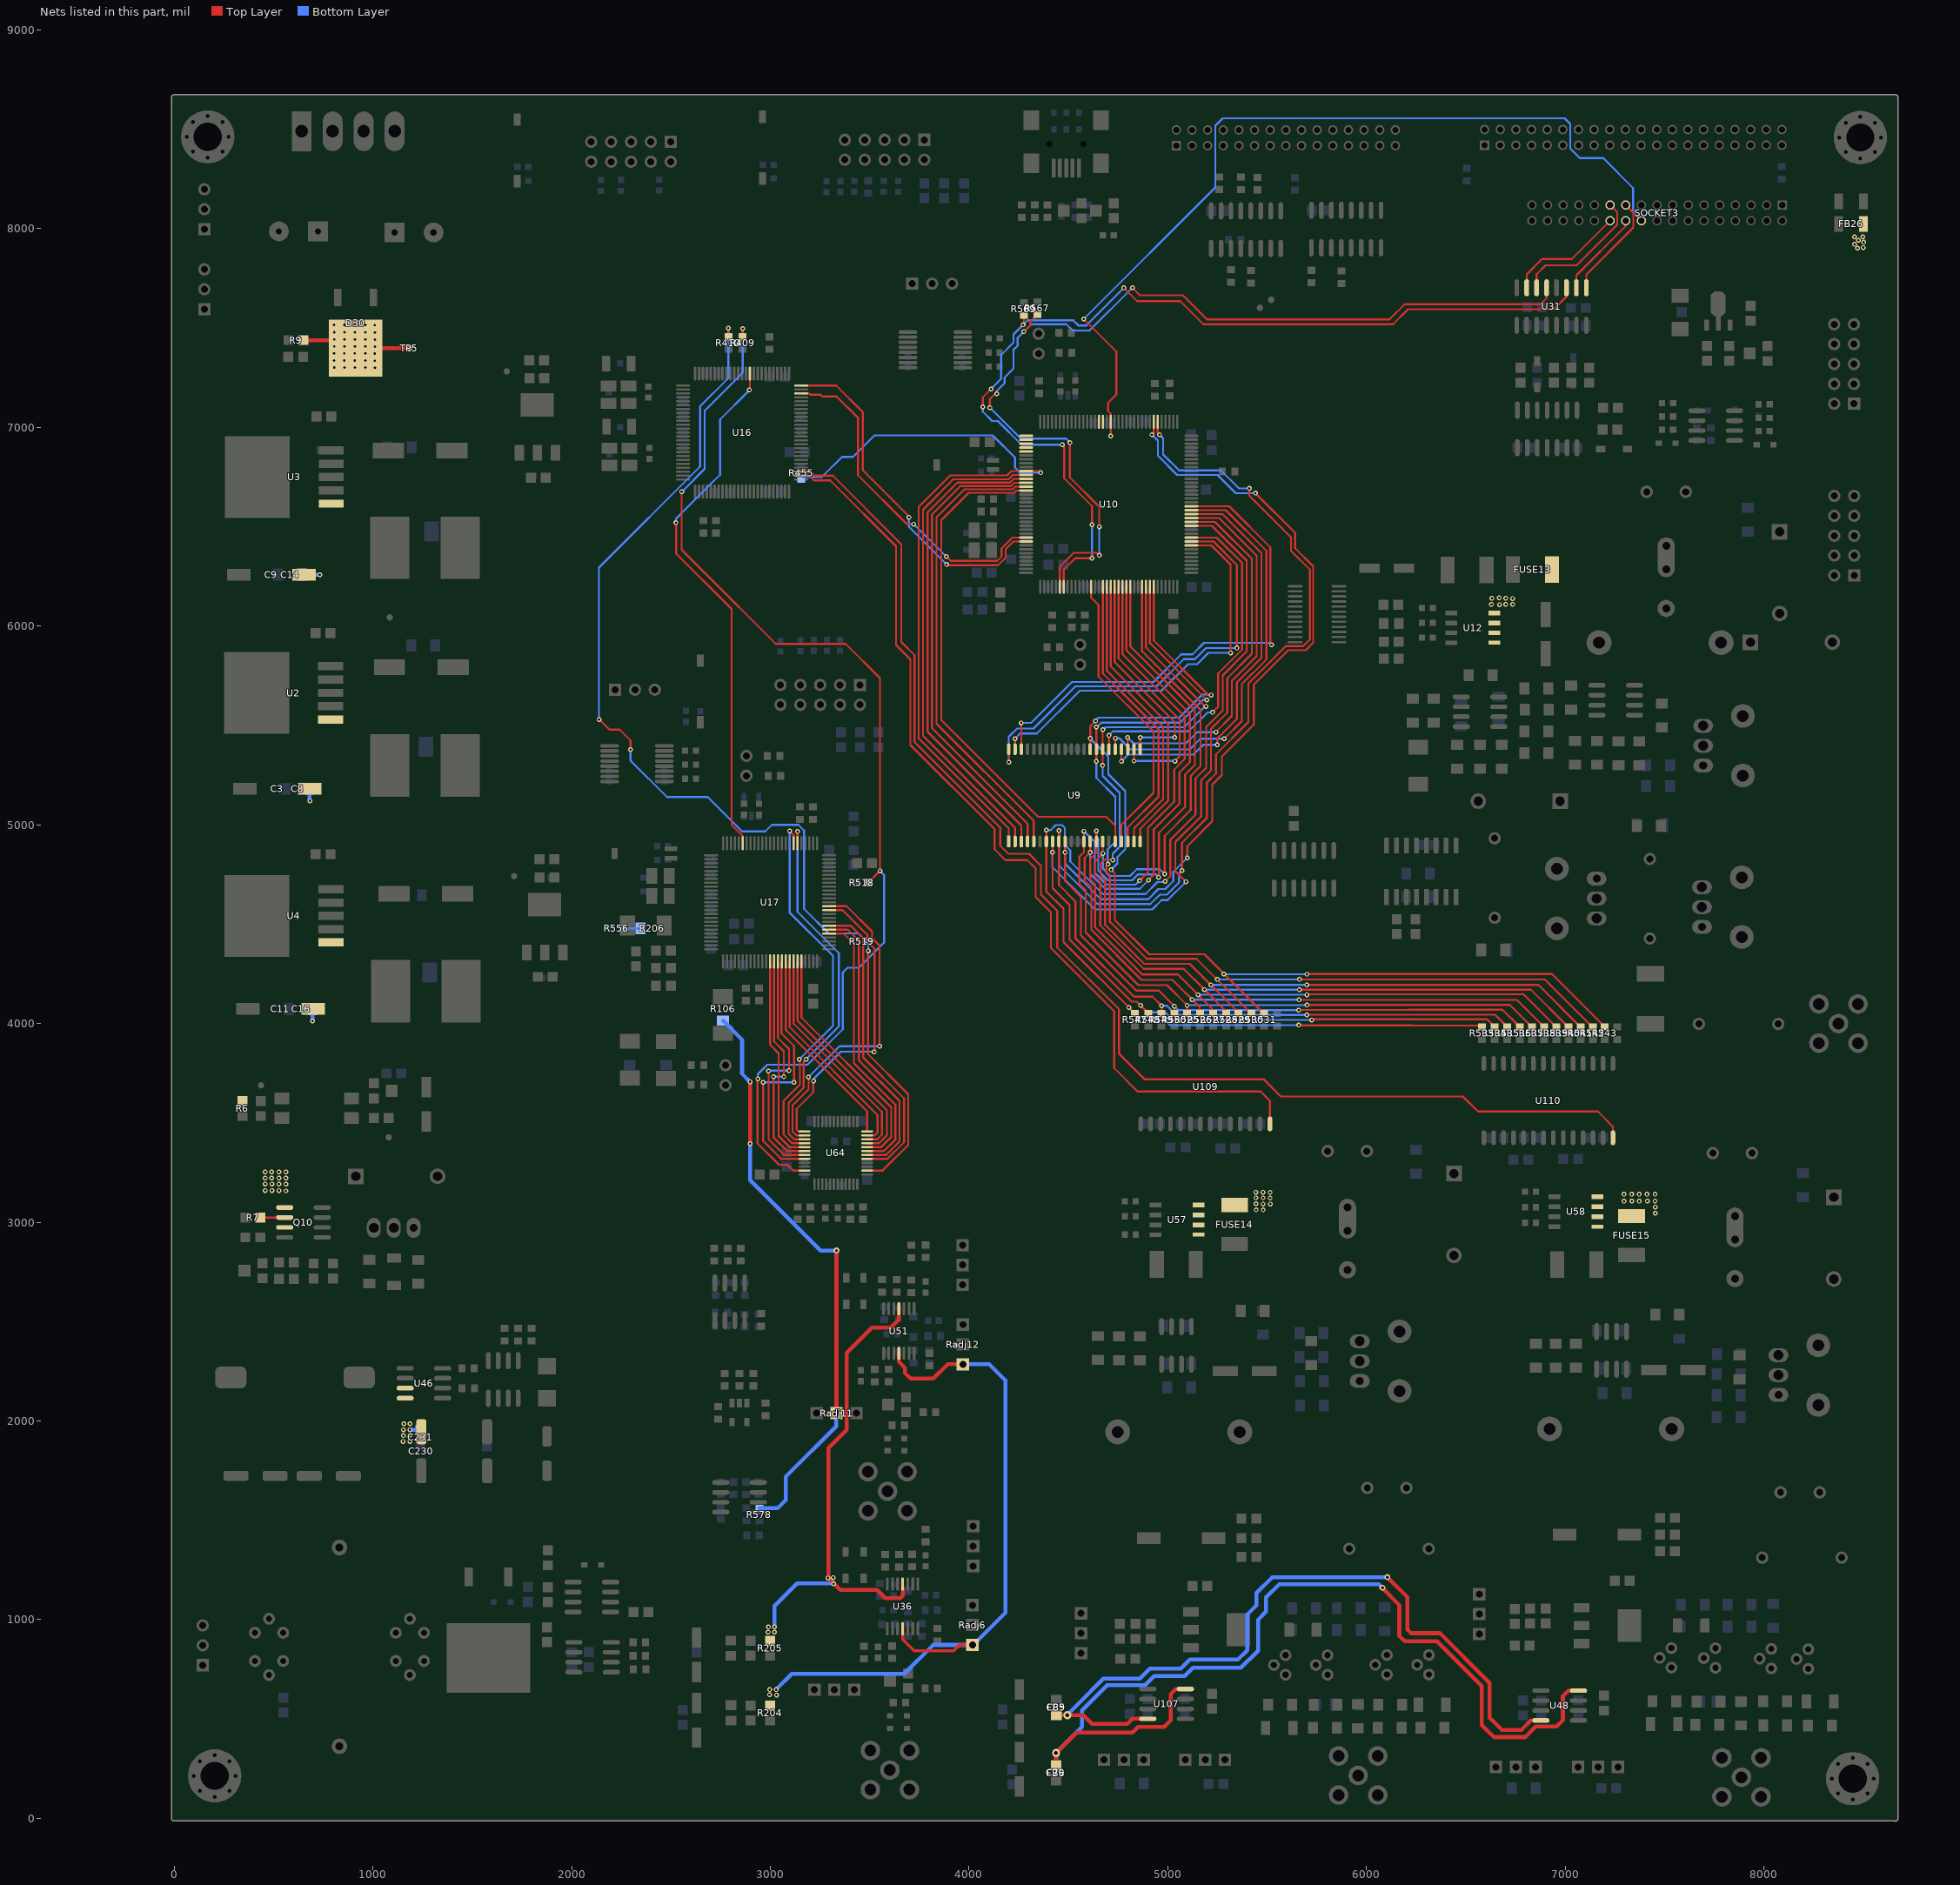
[diagram p0: the nets of this part, all layers, seen from the top]
# Altium PCB MISC82309.PcbDoc (part 6 of 14)
Units mil, origin at the board's own origin, x right, y up, seen from the top; angles counter-clockwise.
Board outline 8687.03 x 8687.86 mil, 4 copper layers (Top Layer, GND, POWER, Bottom Layer); 747 components, 583 nets, 2530 pads, 1834 vias.

## Via types
v1: diameter 24, hole 12, Top Layer to Bottom Layer, 1799 vias
v2: diameter 30, hole 15, Top Layer to Bottom Layer, 26 vias
v3: diameter 40, hole 20, Top Layer to Bottom Layer, 9 vias

## Nets (pads, with @x,y where several pads share a name; then routed paths per layer and width w, separated by ;. In a path a pad name is that pad's centre, name@x,y a point inside that pad or via, vN(x,y) a via of type N, cw(c..) or ccw(c..) an arc to the next point about the centre after c; other vN are vias at no path point) (continued)
DAC_+12V: C89.2 FB5.2 U48.8 U107.8 | length 3887.1
  Top Layer w20: FB5.2@4439,519.61 v3(4494.61,519.61) ; v3@4499,519.61 4575.39,519.61 4619,476 4797,476 4823,502 U107.8@4895,502 ; v2(6105,1214) 6205,1114 6205,951 6224,932 6370,932 6620,682 6620,507 6648,479 ; 6638,489 6648,479 ; U48.8@6877.51,493 6827,493 6780,446 6681,446 6648,479
  Bottom Layer w20: C89.2@4450,520 4450.39,519.61 C89.2@4456,519.61 ; C89.2@4456,520 4493,520 4523.5,550.5 4550.5,577.5 4676,703 4859,703 4910,754 5066,754 5111,799 5353,799 5400,846 5400,1026 5446,1072 5446,1134 5526,1214 v2(6105,1214)
DAC_-12V: C79.2 FB6.2 U48.4 U107.4 | length 4832.5
  Top Layer w20: FB6.2@4438,266.39 v3@4438,328 ; v3@4438.5,328.5 4542,432 4822,432 4851,461 4982,461 5014,493 5014,625 5039,650 U107.4@5085,650 ; v2(6080,1161) 6080,1159 6165,1074 6165,918 6192,891 6355,891 6580,666 6580,470 6641,409 6798,409 6852,463 6957,463 6988,494 6988,616 7015,643 U48.4@7066.49,643
  Bottom Layer w20: C79.2@4435,278 C79.2@4438,281 ; C79.2@4439,277 4439,331 4569,461 4569,544 4696,671 4885,671 4931,717 5085,717 5126,758 5368,758 5454,844 5454,1000 5494,1040 5494,1112 5561,1179 6062,1179 v2(6080,1161)
  other v3: 4438,329
DAC_CLK_A: U16.52 U109.28 | length 4718.4
  Top Layer w10: U16.52@3155.24,6757.46 3196,6757.46 3220.03,6733.44 3301,6733.44 3633,6401.44 3633,5905 3705,5833 3705,5402 4128,4979 4128,4877 4182,4823 4293,4823 4335,4781 4335,4637 4412,4560 4412,4380 4730,4062 4730,3776 4848,3658 5467,3658 5514,3611 U109.28@5514,3515
DAC_CLK_B: U16.53 U110.28 | length 6426.9
  Top Layer w10: U16.53@3155.24,6777.15 3200.85,6777.15 3221,6757 3314,6757 3659,6412 3659,5920 3726,5853 3726,5417 4157,4986 4157,4895 4198,4854 4302,4854 4362,4794 4362,4650 4444,4568 4444,4383 4755,4072 4755,3848 4883,3720 5482,3720 5569,3633 6485,3633 6561,3557 7164,3557 7240,3481 U110.28@7240,3424.99
DC-IN: C3.1 C8.2 C9.1 C11.1 C14.2 C16.2 C230.2 C231.2 D30.4 FB26.1 FUSE13.1 FUSE14.1 FUSE15.1 Q10.1 Q10.2 Q10.3 R6.2 R7.2 R9.2 TP5.1 U2.1 U3.1 U4.1 U12.5 U12.6 U12.7 U12.8 U46.7 U46.8 U57.5 U57.6 U57.7 U57.8 U58.5 U58.6 U58.7 U58.8 | length 778.8
  Top Layer w10: R7.2@433.5,3024 Q10.2@556.51,3024
  Top Layer w20: R9.2@650.5,7439 D30.4@887,7439 ; D30.4@1012,7404 1017,7399 TP5.1@1183,7399
  Bottom Layer w20: C14.2@644,6259 v1@734,6259 ; v1@682,5126 C8.2@682,5181 ; v1@697,4018 C16.2@697,4068 ; v1@1188,1956 1238.5,1956 C231.2@1239,1956.5
  other v1: 1152,1897 1187,1897 1154,1926 1187,1929 1153,1956 1187,1956 1156,1986 1187,1986 7453,3045 5445,3062 5480,3062 7453,3077 5480,3092 5516,3092 5444,3094 7296,3106 7372,3106 7335,3107 7413,3107 7452,3107 5515,3122 5443,3123 5480,3123 7295,3141 7334,3141 7372,3141 7412,3141 7452,3141 5515,3150 5443,3151 5479,3151 562,3158 459,3160 492,3160 528,3160 527,3192 562,3192 459,3193 492,3193 459,3223 491,3223 527,3223 562,3223 459,3253 491,3253 527,3253 562,3253 697,4013 683,5121 6669,6108 6629,6109 6736,6109 6701,6110 6735,6139 6631,6140 6701,6140 6668,6142 733,6258 1011,7300 806,7301 857,7301 910,7301 963,7301 1010,7335 805,7336 856,7336 909,7336 962,7336 1010,7371 805,7372 856,7372 909,7372 962,7372 1011,7406 806,7407 857,7407 910,7407 963,7407 1011,7441 806,7442 857,7442 910,7442 963,7442 1011,7478 806,7479 857,7479 910,7479 963,7479 1010,7515 805,7516 856,7516 909,7516 962,7516 8471,7902 8499,7905 8456,7921 8501,7932 8475,7941 8456,7959 8497,7959
DET+12V: R204.2 Radj6.3 Radj12.3 U36.4 U51.4 | length 3610.8
  Top Layer w16: U36.4@3667,953.8 3667,900 3723,844 3923,844 3952,873 Radj6.3@4015,873
  Top Layer w20: U51.4@3647,2340.8 3647,2298 3678,2267 3678,2241 3706,2213 3820,2213 3892,2285 Radj12.3@3969,2285
  Bottom Layer w20: v1@3030.5,649.5 3108,727 3674,727 3820,873 Radj6.3@4017,873 4021,873 4183,1035 4183,2204 4102,2285 Radj12.3@3969,2285
  other v1: 3031,621 2996,622 2997,648 3030,648
DET-12V: R205.2 U36.11 U51.11 | length 2465.2
  Top Layer w20: v1@3320,1182 3352,1150 3538,1150 3579,1109 3654,1109 3666,1121 U36.11@3666,1161 ; v1@3320.5,1182.5 3292,1211 3292,1863 3385,1956 3385,2343 3511,2469 3606,2469 3647,2510 U51.11@3647,2565.2
  Bottom Layer w20: v1(3021,964) 3021,1069 3134,1182 v1@3316,1182
  other v1: 2989,938 3021,938 2991,963 3319,1181 3290,1210 3317,1212
DET_D0: U17.61 U64.37 | length 1548
  Top Layer w10: U64.37@3172.52,3457.27 3142.73,3457.27 3133,3467 3133,3571 3216,3654 3216,3712 v1(3217,3711) ; U17.61@3296.24,4570.63 3363.37,4570.63 3489,4445 3489,4412 3524,4377 v1@3524,3864 ; v1(3523,3857) 3524,3858 v1@3524,3864 ; v1@3523,3863 v1@3524,3864
  Bottom Layer w10: v1(3217,3711) 3217,3720 3355,3858 3524,3858 v1(3523,3857)
DET_D1: U17.62 U64.38 | length 1659.4
  Top Layer w10: U64.38@3172.52,3437.58 3131.42,3437.58 3112,3457 3112,3588 3193,3669 3193,3729 v1(3192,3730) ; U17.62@3296.24,4590.32 3384.68,4590.32 3512,4463 3512,4431 3550,4393 v1(3550,3886)
  Bottom Layer w10: v1(3192,3730) 3348,3886 v1(3550,3886)
DET_D2: U17.81 U64.39 | length 1862
  Top Layer w10: U17.81@3136.8,4907.24 3136.8,4965.8 v1(3137,4966) ; U64.39@3172.52,3417.9 3120.1,3417.9 3092,3446 3092,3601 3168,3677 3168,3808 v1(3180,3820)
  Bottom Layer w10: v1(3137,4966) 3137,4562 3345,4354 3345,3985 v1(3180,3820)
DET_D3: U17.82 U64.40 | length 1916.8
  Top Layer w10: v1(3097,4969) 3117.11,4948.89 U17.82@3117.11,4907.24 ; v1(3146,3820) 3149,3817 3149,3693 3067,3611 3067,3441 3109.79,3398.21 U64.40@3172.52,3398.21
  Bottom Layer w10: v1(3097,4969) 3097,4559 3315,4341 3315,3989 v1(3146,3820)
DET_D4: U17.38 U64.41 | length 1050.3
  Top Layer w10: U17.38@2999,4312.76 2999,3893 3042,3850 3042,3630 3042,3433.53 3097,3378.53 U64.41@3172.52,3378.53
DET_D5: U17.39 U64.42 | length 1147
  Top Layer w10: v1@3016,3737 v1(3016,3733) 3016,3680 3016,3426.84 3084,3358.84 U64.42@3172.52,3358.84 ; U17.39@3018.68,4312.76 3018.68,3910.32 3068,3861 v1(3068,3733)
  Bottom Layer w10: v1(3016,3733) v1(3068,3733)
DET_D6: U17.40 U64.43 | length 1234.3
  Top Layer w10: v1(2991,3761) 2991,3717 2991,3417.16 3069,3339.16 U64.43@3172.52,3339.16 ; U17.40@3038.37,4312.76 3038.37,3927.63 3094,3872 v1(3094,3763)
  Bottom Layer w10: v1(2991,3761) 2993,3763 v1(3094,3763)
DET_D7: U17.41 U64.44 | length 1332.2
  Top Layer w10: v1(2964,3704) 2964,3684 2964,3409.47 3054,3319.47 U64.44@3172.52,3319.47 ; U17.41@3058.06,4312.76 3056.28,4310.98 3056.28,3950.72 3119,3888 3119,3705 v1(3120,3704)
  Bottom Layer w10: v1(2964,3704) v1(3120,3704)
DET_D8: U17.42 U64.24 | length 1028.8
  Top Layer w10: U17.42@3077.74,4312.76 3077.74,3968.26 3487.48,3558.52 U64.24@3487.48,3457.27 U64.24@3490,3459.79
DET_D9: U17.43 U64.23 | length 1104.8
  Top Layer w10: U17.43@3099,4311.18 U17.43@3097.43,4312.76 3097.43,3981.57 3540,3539 3540,3452 3525.58,3437.58 U64.23@3487.48,3437.58
DET_D10: U17.44 U64.22 | length 1140.1
  Top Layer w10: U17.44@3117.11,4312.76 3117.11,3999.89 3562,3555 3562,3441 3538.9,3417.9 U64.22@3487.48,3417.9
DET_D11: U17.45 U64.21 | length 1177.2
  Top Layer w10: U17.45@3136.8,4312.76 3136.8,4014.2 3587,3564 3587,3438 3547.21,3398.21 U64.21@3487.48,3398.21
DET_D12: U17.46 U64.20 | length 1216.1
  Top Layer w10: U17.46@3158.26,4310.98 U17.46@3156.48,4312.76 3156.48,4030.52 3609,3578 3609,3429 3558.53,3378.53 U64.20@3487.48,3378.53
DET_D13: U17.55 U64.19 | length 1383.9
  Top Layer w10: U17.55@3296.24,4452.52 3369.48,4452.52 3420,4402 3420,3800 3630,3590 3630,3416 3572.84,3358.84 U64.19@3487.48,3358.84
DET_D14: U17.56 U64.18 | length 1458.3
  Top Layer w10: U17.56@3296.24,4472.2 3390.8,4472.2 3445,4418 3445,3816 3650,3611 3650,3406 3583.16,3339.16 U64.18@3487.48,3339.16
DET_D15: U17.57 U64.17 | length 1529.4
  Top Layer w10: U17.57@3296.24,4491.89 3405.11,4491.89 3468,4429 3468,3828 3673,3623 3673,3402 3590.47,3319.47 U64.17@3487.48,3319.47
DETECT-RST: U16.86 U17.95 | length 2654
  Top Layer w10: v1@2526,6520 2526,6365 2805,6086 2805,5000 2861.2,4943.8 U17.95@2861.2,4907.24 ; v1@2897.37,7190.37 U16.86@2897.37,7271.24
  Bottom Layer w10: v1(2525,6520) 2525,6540 2568,6583 2568,6583.47 2690.53,6706 2691,6706 2747,6762 2747,7040 v1(2895,7188)
DROP-CH_A: R206.1 R556.1 | length 82.7
  Bottom Layer w10: R556.1@2258.5,4479 2337,4479 R206.1@2340,4476
DROP-CH_B: R106.1 R578.1 Radj11.2 | length 2948.4
  Top Layer w20: v1(2898,3396) v1(2898,3707) ; Radj11.2@3333,2039 v2(3333,2858)
  Bottom Layer w20: R106.1@2762,4015 2858,3919 2858,3747 v1(2898,3707) ; v1(2898,3396) 2898,3212 3253,2857 v2@3332,2857 ; R578.1@2945,1560.5 3036.5,1560.5 3077,1601 3077,1719 3331,1973 Radj11.2@3331,2036
DROP_A: U10.27 U16.73 | length 1721.6
  Top Layer w10: U16.73@3155.24,7170.85 3195.15,7170.85 3202,7164 3253,7164 3261,7156 3333,7156 3440,7049 ; 3441,7049 3441,6760 3688,6513 v1(3721,6513) ; v1(3885,6350) v1@3886.5,6348.5 ; v1@3887,6349 3908,6328 4141.51,6328 4164,6350.49 4164,6391.04 4218.64,6445.68 U10.27@4287.65,6445.68
  Bottom Layer w10: v1@3723,6514 3723,6512 v1(3885,6350)
DROP_B: U10.28 U16.75 | length 1803.5
  Top Layer w10: U16.75@3155.24,7210.22 3331.78,7210.22 3464,7078 ; 3465,7078 3465,6785 v1@3703,6547 ; v1(3887,6310) 3887,6308 3885,6306 4146,6306 4184,6344 4184,6387 4222.99,6425.99 U10.28@4287.65,6425.99
  Bottom Layer w10: v1@3705,6548 3697,6540 3697,6500 3885,6312 3885,6306 3887,6308 v1(3887,6310)
  other v1: 3698,6547
ENC_A: R409.2 R518.2 U64.47 | length 5687.8
  Top Layer w10: v1(2554,6676) 2554,6384 2663,6275 3028,5910 3380,5910 3552,5738 v1(3552,4768.5) R518.2@3492.5,4709 ; R409.2@2861,7455.5 v1(2861,7497) ; v1@2936,3716 2936,3397 3044,3289 3086,3289 3114.58,3260.42 U64.47@3172.52,3260.42
  Bottom Layer w10: v1@2554.5,6675.5 2670,6791 2670,7084 2861,7275 v1(2861,7497) ; v1@2937,3717 v1(2937,3722) 2937,3745 2985,3793 3186.94,3793 3365,3971.06 3365,4257 3389,4281 3446,4281 3572,4407 3572,4748.5 v1(3552,4768.5)
ENC_B: R410.2 R519.2 U64.14 | length 5783.3
  Top Layer w10: v1@2140,5529 2190,5479 2242,5479 2297,5424 v1(2297,5379) ; v1(2789,7499) 2790,7498 R410.2@2790,7456.5 ; U64.14@3487.48,3260.42 3565.42,3260.42 3694,3389 3694,3644 3492,3846 3492,4365 v1(3493,4366)
  Bottom Layer w10: v1(2138,5529) 2138,6294 2647,6803 2647,7106 2789,7248 v1(2789,7499) ; v1(2297,5379) 2297,5323 2480,5140 2685,5140 2858,4967 2975,4967 3008,5000 3141,5000 3170,4971 3170,4577 3293,4454 3443.88,4454 3483.88,4414 R519.2@3492.5,4414 3493,4413.5 v1(3493,4366)
ENCODE_PA: R567.2 U10.42 U31.5 | length 4915
  Top Layer w10: v1(4105,7099) 4105,7143 4131,7169 v1(4139,7169) ; v1@4274,7480 v1(4276,7482) 4308,7514 4308,7533 R567.2@4332,7557 ; U10.42@4456.94,6197.65 4456.94,6298.94 4527,6369 4642,6369 v1(4655,6356) ; v1@4507,6918 4507,6749 4655,6601 v1(4655,6500) ; v1(4822,7703) 4860,7665 5076,7665 5198,7543 6115,7543 6192,7620 6876,7620 6906,7650 U31.5@6906,7702.49
  Bottom Layer w10: v1(4105,7099) 4261,6943 4488,6943 v1(4508,6923) ; v1(4139,7169) 4139,7183 4178.5,7222.5 4178.5,7250.5 4224,7296 4224,7391 4245,7412 4245,7451 v1(4276,7482) 4313,7519 4490,7519 4522,7487 4606,7487 v1(4822,7703) ; v1@4659,6352 v1(4655,6356) v1(4655,6500) v1@4659,6496
ENCODE_PB: R569.2 U10.43 U31.3 | length 4953.8
  Top Layer w10: v1(4069,7103) 4069,7151 v1(4111,7193) ; v1@4272,7509 v1(4272,7516) ; v1@4274,7516 4276,7518 R569.2@4276,7564.5 ; v1(4469,6913) 4479,6903 4479,6744 4619,6604 v1(4619,6510) ; U10.43@4476.62,6197.65 4476.62,6284.62 4534,6342 v1(4619,6342) ; v1(4779,7702) 4846,7635 5063,7635 5179,7519 6133,7519 6209,7595 6943,7595 7006,7658 U31.3@7006,7702.49
  Bottom Layer w10: v1(4069,7103) 4069,7079 4116,7032 4145,7032 4264,6913 4321,6913 v1(4469,6913) ; v1@4111,7194 4161,7244 4161,7364 4224,7427 4224,7468 v1(4272,7516) ; v1@4275.5,7512.5 4272,7509 v1(4272,7516) ; v1(4619,6342) v1(4619,6510) ; v1(4779,7702) 4590,7513 4550,7513 4524,7539 4295,7539 v1(4272,7516)
ENCODER_TRACK_AN: SOCKET3.24 U31.7 | length 599.3
  Top Layer w10: U31.7@6806,7702.49 6806,7770 6883,7847 7032.6,7847 SOCKET3.24@7225.86,8040.26
ENCODER_TRACK_AP: SOCKET3.23 U31.6 | length 690.6
  Top Layer w10: U31.6@6856,7702.49 6856,7771 6901,7816 7057,7816 7261.48,8020.48 7261.48,8083.38 SOCKET3.23@7225.86,8119
ENCODER_TRACK_BN: SOCKET3.21 U31.1 | length 530.6
  Top Layer w10: U31.1@7106,7702.49 7106,7769 7343,8006 7343,8080.6 SOCKET3.21@7304.6,8119
ENCODER_TRACK_BP: SOCKET3.22 U31.2 | length 440.7
  Top Layer w10: U31.2@7056,7702.49 7056,7765 7304.6,8013.6 SOCKET3.22@7304.6,8040.26
EPRINT-RST: SOCKET3.20 U10.126 | length 4442.7
  Top Layer w10: v1(4577,7545) 4741,7381 4741,7165 4700,7124 4700,7081 4712.84,7068.16 U10.126@4712.84,7028.35 4712.84,6957.16 v1(4713,6957)
  Bottom Layer w10: v1(4577,7545) 5239,8207 5239,8518 5276,8555 6997,8555 7025,8527 7025,8403 7073,8355 7191,8355 7342,8204 7342,8081.6 SOCKET3.20@7383.34,8040.26
FSMC_A0: R455.2 U9.1 U10.10 | length 3953.5
  Top Layer w10: U9.1@4200,4916 4200,4982 3747,5435 3747,6600 3905,6758 4191,6758 4213.32,6780.32 U10.10@4287.65,6780.32 4351.68,6780.32 v1(4360,6772)
  Bottom Layer w10: R455.2@3163,6751 3260,6751 3361,6852 3416,6852 3524,6960 4119,6960 4231,6848 4231,6798 4257,6772 v1(4360,6772)
FSMC_A1: U9.2 U10.11 | length 2454
  Top Layer w10: U9.2@4231.5,4916 4231.5,4985.5 3768,5449 3768,6586 3921,6739 4198.83,6739 4220.47,6760.64 U10.11@4287.65,6760.64
FSMC_A2: U9.3 U10.12 | length 2417.3
  Top Layer w10: U9.3@4262.99,4916 4262.99,4996.01 3792,5467 3792,6573 3941,6722 4205.88,6722 4224.83,6740.95 U10.12@4287.65,6740.95
FSMC_A3: U9.4 U10.13 | length 2385.5
  Top Layer w10: U10.13@4287.65,6721.27 4229.18,6721.27 4212.92,6705 3957,6705 3813,6561 3813,5487 4294.49,5005.51 U9.4@4294.49,4916
FSMC_A4: U9.5 U10.14 | length 2349.6
  Top Layer w10: U10.14@4287.65,6701.58 4233.54,6701.58 4219.96,6688 3977,6688 3836,6547 3836,5509 4325.98,5019.02 U9.5@4325.98,4916
FSMC_A5: U9.18 U10.15 | length 2670.5
  Top Layer w10: U10.15@4287.65,6681.9 4287.54,6682 4238,6682 4227,6671 4181.94,6671 3998,6671 3860,6533 3860,5527 4347,5040 4691,5040 4735.43,4995.57 U9.18@4735.43,4916
FSMC_A6: U9.19 U10.50 | length 1478.3
  Top Layer w10: U10.50@4614.42,6197.65 4614.42,6143.58 4652,6106 4652,5746 4928,5470 4928,5161 4766.93,4999.93 U9.19@4766.93,4916
FSMC_A7: U9.20 U10.53 | length 1461.5
  Top Layer w10: U10.53@4673.47,6197.65 4673.47,5761.53 4775,5660 4953,5482 4953,5141 4798.43,4986.43 U9.20@4798.43,4916
FSMC_A8: U9.21 U10.54 | length 1460.1
  Top Layer w10: U10.54@4693.16,6197.65 4693.16,5775.84 4977,5492 4977,5129 4829.92,4981.92 U9.21@4829.92,4916
FSMC_A9: U9.22 U10.55 | length 1459.6
  Top Layer w10: U10.55@4712.84,6197.65 4712.84,5798.16 5002,5509 5002,5121 4861.42,4980.42 U9.22@4861.42,4916
FSMC_A10: U9.23 U10.56 | length 1113.4
  Top Layer w10: U10.56@4732.53,6197.65 4732.53,5819.47 5036,5516 v1@5036,5442 ; U9.23@4861.42,5380.57 v1(4861.42,5439.42)
  Bottom Layer w10: v1(4861.42,5439.42) 4896,5439.42 v1(5034.58,5439.42)
FSMC_A11: U9.24 U10.57 | length 1281.1
  Top Layer w10: U10.57@4752.21,6197.65 4752.21,5837.79 5060,5530 5060,5344 v1(5036,5320) ; v1(4829.92,5321.08) U9.24@4829.92,5380.57
  Bottom Layer w10: v1(4829.92,5321.08) 5034.92,5321.08 v1(5036,5320)
FSMC_A12: U9.25 U10.87 | length 1923.2
  Top Layer w10: U9.25@4798.43,5380.57 v1(4798.43,5439.57) ; U10.87@5118.35,6544.1 5257.9,6544.1 5447,6355 5447,5849 5322,5724 5322,5548 v1@5240,5466
  Bottom Layer w10: v1(4798.43,5439.57) 4828,5410 5092,5410 5148,5466 5244,5466 v1(5243,5467)
FSMC_A13: U9.26 U10.88 | length 2076.6
  Top Layer w10: v1(4766.93,5319.07) U9.26@4766.93,5380.57 ; U10.88@5118.35,6563.79 5275.21,6563.79 5471,6368 5471,5840 5347,5716 5347,5532 5249,5434 v1(5249,5402)
  Bottom Layer w10: v1(4766.93,5319.07) 4800.86,5353 5129,5353 5178,5402 v1(5249,5402) v1@5256,5402
FSMC_A14: U9.27 U10.89 | length 2143.7
  Top Layer w10: U9.27@4735.43,5380.57 v1@4735.43,5436 ; U10.89@5118.35,6583.47 5291.53,6583.47 5496,6379 5496,5832 5373,5709 5373,5522 v1(5284,5433)
  Bottom Layer w10: v1(4737,5436) 4755,5436 4811,5380 5111,5380 5164,5433 v1(5284,5433)
FSMC_A15: U9.42 U10.90 | length 2538.4
  Top Layer w10: U9.42@4262.99,5380.57 v1(4262.99,5512.99) ; U10.90@5118.35,6603.16 5308.84,6603.16 5516,6396 5516,5912 v1(5522,5906)
  Bottom Layer w10: v1(4262.99,5512.99) 4311.99,5512.99 4518,5719 4928,5719 5067,5858 5124,5858 5182,5916 5512,5916 v1(5522,5906)
FSMC_A16: U9.43 U10.80 | length 1998.7
  Top Layer w10: U9.43@4231.5,5380.57 v1(4231.5,5433.5) ; U10.80@5118.35,6406.31 5219.69,6406.31 5316,6310 v1(5316,5865)
  Bottom Layer w10: v1(4231.5,5433.5) 4257,5459 4341,5459 4557,5675 4968,5675 5102,5809 5148,5809 5204,5865 v1(5316,5865)
FSMC_A17: U9.44 U10.81 | length 2223.2
  Top Layer w10: v1(4200,5315) U9.44@4200,5380.57 ; U10.81@5118.35,6425.99 5230.01,6425.99 5348,6308 v1(5348,5890)
  Bottom Layer w10: v1(4200,5315) 4200,5443 4242,5485 4324,5485 4536,5697 4944,5697 5081,5834 5136,5834 5192,5890 v1(5348,5890)
FSMC_A18: U9.28 U10.82 | length 1760.7
  Top Layer w10: U9.28@4703.94,5380.57 v1@4703.94,5450 ; U10.82@5118.35,6445.68 5246.32,6445.68 5374,6318 5374,5882 5253,5761 5253,5594 v1(5225,5566)
  Bottom Layer w10: v1(4704,5450) 4724,5470 5105,5470 5201,5566 v1(5225,5566)
FSMC_A19: U10.2
FSMC_A20: U10.3
FSMC_A21: U10.4
FSMC_A22: U10.5
FSMC_A23: U10.1
FSMC_A24: U10.128
FSMC_A25: U10.129
FSMC_D0: R533.2 R547.2 U9.7 U10.85 | length 5928.9
  Top Layer w10: v1(4388.98,4974.02) U9.7@4388.98,4916 4388.98,4693 4389,4664 4475,4578 4475,4410.5 R547.2@4835,4050.5 ; v1(4986,4715) 5013,4742 5013,4924 5140,5051 5140,5234 5193,5287 5193,5492 5276,5575 5276,5752 5397,5873 5397,5908 ; U10.85@5118.35,6504.73 5221.27,6504.73 5397,6329 5397,5908 ; 5397,5901 5397,5908 ; v1(5659,3992) 5660,3991 6234,3991 6235,3990 6574,3990 R533.2@6581,3983
  Bottom Layer w10: v1(4388.98,4974.02) 4411.02,4974.02 4436,4999 4468,4999 4482,4985 4482,4899 4509.03,4871.97 ; 4509,4871.94 4509,4816 4673,4652 4888,4652 4948,4712 4983,4712 v1(4986,4715) ; v1(4804,4081) 4851,4034 4969,4034 5011,3992 v1(5659,3992)
FSMC_D1: R534.2 R548.2 U9.8 U10.86 | length 5986
  Top Layer w10: v1(4420,4862) v1@4420.47,4862 ; U9.8@4420.47,4916 v1@4420.47,4862 ; R548.2@4896,4058 4844,4110 4818,4110 4506,4422 4506,4596 4420.47,4681.53 v1@4420.47,4862 ; v1(5091,4714) 5038,4767 5038,4913 5168,5043 5168,5224 5217,5273 5217,5483 5299,5565 5299,5737 5423,5861 5423,6339 5237.58,6524.42 U10.86@5118.35,6524.42 ; v1(5725,4018) 5725,4020 5723,4022 6606,4022 R534.2@6645,3983
  Bottom Layer w10: v1(4420,4862) 4420,4788 4634,4574 4922,4574 4969,4621 4999,4621 5091,4713 v1(5091,4714) ; v1(4863,4091) 4898,4056 4987,4056 5025,4018 v1(5725,4018)
FSMC_D2: R535.2 R549.2 U9.9 U10.114 | length 6988.6
  Top Layer w10: v1(4451.97,4970.97) U9.9@4451.97,4916 4451.97,4698.03 4535,4615 4535,4430 4830,4135 4923,4135 4970,4088 R549.2@4970,4053 ; U10.114@4949.06,7028.35 4949.06,6972.94 v1(4959,6963) ; v1(5072,4770) 5072,4910 5196,5034 5196,5211 5243,5258 5243,5354 5406,5517 5406,5711 5594,5899 5681,5899 5714.84,5932.84 5714.84,6284.16 5620,6379 5620,6447 5410,6657 v1(5410,6693) ; v1(5700,4043) 5701,4044 6208,4044 6647,4044 R535.2@6708,3983
  Bottom Layer w10: v1(4451.97,4970.97) 4451.97,4796.03 4647,4601 4912,4601 4960,4649 4995,4649 5057,4711 5057,4755 v1(5072,4770) ; v1(4959,6963) 4977,6945 4977,6864 5057,6784 5267,6784 5358,6693 v1(5410,6693) ; v1(4969,4089) 4996,4089 5042,4043 v1(5700,4043)
FSMC_D3: R536.2 R550.2 U9.10 U10.115 | length 6829.5
  Top Layer w10: U9.10@4483.47,4916 v1@4483.47,4863 ; v1(4484,4862.47) v1@4483.47,4863 ; v1(4920,6963) 4929.38,6972.38 U10.115@4929.38,7028.35 ; R550.2@5034,4050.5 5034,4087 4955,4166 4841,4166 4563,4444 4563,4638 4483.47,4717.53 v1@4483.47,4863 ; v1(5098,4833) 5098,4892 5224,5018 5224,5202 5272,5250 5272,5343 5433,5504 5433,5706 5606,5879 5694.04,5879 5731.84,5916.8 5731.84,6301.16 5641,6392 5641,6469 v1(5441,6669) ; v1(5659,4067) 5660,4067 5662,4069 6215,4069 6216,4070 6684,4070 R536.2@6771,3983
  Bottom Layer w10: v1(4484,4862.47) 4484,4804 4662,4626 4902,4626 4953,4677 4987,4677 5028,4718 5028,4763 v1(5098,4833) ; v1(4920,6963) 4950,6933 4950,6858 5047,6761 5250,6761 5342,6669 v1(5441,6669) ; v1(5033,4087) 5053,4067 v1(5659,4067)
FSMC_D4: R525.2 R537.2 U9.13 U10.58 | length 5210.9
  Top Layer w10: v1(4577.95,4967.95) U9.13@4577.95,4916 4577.95,4861.95 ; 4578,4862 4577.95,4861.95 ; U10.58@4771.9,6197.65 4771.9,5859.1 5085,5546 5085,5331 5032,5278 5032,5117 4900,4985 4900,4761 v1(4858,4719) ; R525.2@5098,4050.5 5098,4091 4996,4193 4852,4193 4587,4458 4587,4670 4555.5,4701.5 4555.5,4839.5 4577.95,4861.95 ; v1(5701,4093) 5702,4094 6187,4094 6721,4094 R537.2@6832,3983
  Bottom Layer w10: v1(4577.95,4967.95) 4633,4912.91 4633,4758 4692,4699 4838,4699 v1(4858,4719) ; v1(5097,4091) 5099,4093 v1(5701,4093)
FSMC_D5: R526.2 R538.2 U9.14 U10.59 | length 5173.3
  Top Layer w10: U9.14@4609.45,4916 4609.45,4861.45 v1(4609,4861) 4582,4834 4582,4719 4615,4686 4615,4472 4867,4220 5024,4220 5160,4084 R526.2@5160,4057 ; U10.59@4791.58,6197.65 4791.58,5878.42 5111,5559 5111,5316 5059,5264 5059,5106 4930,4977 4930,4749 v1(4903,4722) ; v1(5661,4119) 6169,4119 6757,4119 R538.2@6893,3983
  Bottom Layer w10: v1(4609,4861) 4609,4754 4685,4678 4859,4678 v1(4903,4722) ; v1(5123,4120) 5660,4120 v1(5661,4119)
FSMC_D6: R527.2 R539.2 U9.15 U10.60 | length 5381.4
  Top Layer w10: v1(4640.94,4968.94) U9.15@4640.94,4916 4640.94,4858.94 4610,4828 4610,4725 4634,4701 4634,4484 4871,4247 5051,4247 5228,4070 R527.2@5228,4050.5 ; U10.60@4811.27,6197.65 4811.27,5898.73 5136,5574 5136,5302 5087,5253 5087,5091 4956,4960 4956,4738 v1(4954,4736) ; v1(5700,4145) 5700,4146 5701,4147 6790,4147 6954,3983 R539.2@6955,3983
  Bottom Layer w10: v1(4640.94,4968.94) 4640.94,4936.06 4650,4927 4650,4770 4699,4721 4821,4721 4850,4750 4940,4750 v1(4954,4736) ; v1(5152,4145) v1(5700,4145)
FSMC_D7: R528.2 R540.2 U9.16 U10.63 | length 5253
  Top Layer w10: v1@4672.44,4853.44 4633,4814 4633,4737 4660,4710 4660,4494 4879,4275 5080,4275 v1(5184,4171) 5293,4062 R528.2@5293,4050.5 ; v1@4672.44,4856 v1@4672.44,4856.44 ; U9.16@4672.44,4916 v1@4672.44,4856.44 ; v1(4674,4856) 4672.88,4856 v1@4672.44,4856.44 ; U10.63@4870.32,6197.65 4870.32,5873.68 5165,5579 5165,5295 5115,5245 5115,5074 4984,4943 v1(4984,4752) ; v1(5662,4170) 5662,4169 5663,4170 5673,4170 6827,4170 R540.2@7005,3992 ; R540.2@7005.5,3992.5 7015,3983 R540.2@7016,3983
  Bottom Layer w10: v1(4674,4856) 4674,4780.06 4711.06,4743 4810,4743 4844,4777 4959,4777 v1(4984,4752) ; v1(5184,4171) 5185,4170 5661,4170 5662,4169 v1(5662,4170)
FSMC_D8: R529.2 R541.2 U9.29 U10.64 | length 5202.8
  Top Layer w10: v1(4672,5299) U9.29@4672,5380.57 ; U9.29@4672.44,5380.57 4672.44,5475.44 4676,5479 v1(4674,5479) ; v1@4719,4826 4683,4826 4664,4807 4664,4741 4684,4721 4684,4498 4881,4301 5110,4301 5356,4055 R529.2@5356,4050.5 ; U10.64@4890.01,6197.65 4890.01,5892.99 5184,5599 5192,5599 v1(5192,5596) ; R529.2@5353,4049 5354,4050 R529.2@5354,4050.5 ; v1(5699,4194) 5700,4195 6123,4195 6864,4195 7076,3983 R541.2@7077,3983
  Bottom Layer w10: v1@4672.44,5298.56 4672.44,5246.56 4758,5161 4758,4889 4723,4854 v1(4723,4822) ; v1(4674,5479) 4676,5479 4688,5491 5083.12,5491 5191.56,5599.44 5192,5599 v1(5192,5596) ; v1(5217,4194) v1(5699,4194)
FSMC_D9: R530.2 R542.2 U9.30 U10.65 | length 5236.8
  Top Layer w10: v1(4640.94,5319.06) U9.30@4640.94,5380.57 4640.94,5488.94 4644,5492 v1(4641,5492) ; v1@4698,4801 v1(4699,4802) ; v1@4699,4800 4690.5,4791.5 4690.5,4755.5 4709,4737 4709,4512 4895,4326 5144,4326 5419.5,4050.5 R530.2@5422,4050.5 ; U10.65@4909.69,6197.65 4909.69,5915.31 v1(5197.06,5627.94) ; v1(5663,4222) 6106,4222 6897,4222 7136,3983 R542.2@7138,3983
  Bottom Layer w10: v1(4640.94,5319.06) 4640.94,5236.06 4736,5141 4736,4914 4698,4876 v1@4698,4807.38 ; v1(4641,5492) 4644,5492 4666,5514 5062,5514 5175.94,5627.94 v1(5197.06,5627.94) ; v1(5250,4222) v1(5663,4222)
FSMC_D10: R531.2 R543.2 U9.31 U10.66 | length 5468.3
  Top Layer w10: U9.31@4609.45,5380.57 v1(4609.45,5434.55) 4609.45,5495.45 v1(4637,5523) ; v1@4712,4777 4734,4755 4734,4521 4906,4349 5184,4349 5482,4051 R531.2@5485,4051 ; U10.66@4929.38,6197.65 4929.38,5927.62 5202,5655 v1@5219,5655 ; v1(5700,4248) 5698,4248 5699,4249 6933,4249 R543.2@7199,3983
  Bottom Layer w10: v1@4609.45,5439.45 v1(4609.45,5434.55) 4701,5343 4701,5255 4786,5170 4786,4877 4745,4836 4745,4833.94 4747,4831.94 4747,4806 v1(4714.5,4773.5) ; v1@4642,5530 4651,5539 5057,5539 5173,5655 v1@5219,5655 ; v1(5282,4249) 5283,4248 v1(5700,4248)
  other v1: 5219,5653